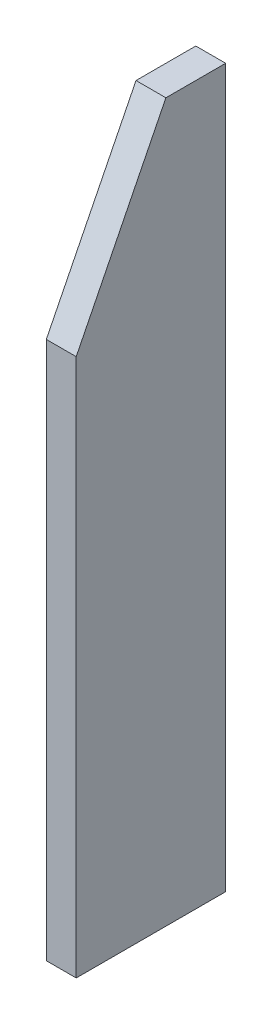
from build123d import *

# Parameters (mm, degrees)
SKETCH_1_W             = 10
SKETCH_1_H             = 240
EXTRUDE_1_DEPTH        = 50
HOLE_WIZARD_M4_2_D     = 3.3
HOLE_WIZARD_M4_2_DEPTH = 15
HOLE_WIZARD_M4_2_TIP   = 0.991420021
HOLE_WIZARD_M4_3_D     = 3.3
HOLE_WIZARD_M4_3_DEPTH = 15
HOLE_WIZARD_M4_3_TIP   = 0.991420021
CHAMFER_1_SIZE         = 30
CHAMFER_1_SIZE2        = 60


with BuildPart() as part:
    # 草图1 → 凸台-拉伸1 (new body)
    with BuildSketch(Plane.XY):
        Rectangle(SKETCH_1_W, SKETCH_1_H)
    extrude(amount=EXTRUDE_1_DEPTH)

    # M4 螺纹孔2
    with Locations(Plane(origin=(0, 0, 0), x_dir=(-1, 0, 0), z_dir=(0, 0, -1))):
        with Locations((0, 97.5), (0, 32.5), (0, -32.5), (0, -97.5)):
            Hole(HOLE_WIZARD_M4_2_D / 2, depth=HOLE_WIZARD_M4_2_DEPTH)
            with Locations((0, 0, -(HOLE_WIZARD_M4_2_DEPTH + HOLE_WIZARD_M4_2_TIP / 2))):  # 118° drill point
                Cone(0, HOLE_WIZARD_M4_2_D / 2, HOLE_WIZARD_M4_2_TIP, mode=Mode.SUBTRACT)

    # M4 螺纹孔3
    with Locations(Plane(origin=(0, -120, 0), x_dir=(-1, 0, 0), z_dir=(0, -1, 0))):
        with Locations((0, -10), (0, -40)):
            Hole(HOLE_WIZARD_M4_3_D / 2, depth=HOLE_WIZARD_M4_3_DEPTH)
            with Locations((0, 0, -(HOLE_WIZARD_M4_3_DEPTH + HOLE_WIZARD_M4_3_TIP / 2))):  # 118° drill point
                Cone(0, HOLE_WIZARD_M4_3_D / 2, HOLE_WIZARD_M4_3_TIP, mode=Mode.SUBTRACT)

    # 倒角1
    chamfer_1_edges = [part.edges().sort_by_distance(p)[0] for p in [
        (0, 120, 50),
    ]]
    chamfer_1_side = [part.faces().sort_by_distance(p)[0] for p in [
        (0, 120, 25),
    ]]
    chamfer(chamfer_1_edges, length=CHAMFER_1_SIZE, length2=CHAMFER_1_SIZE2, reference=chamfer_1_side[0])


solid = part.part
